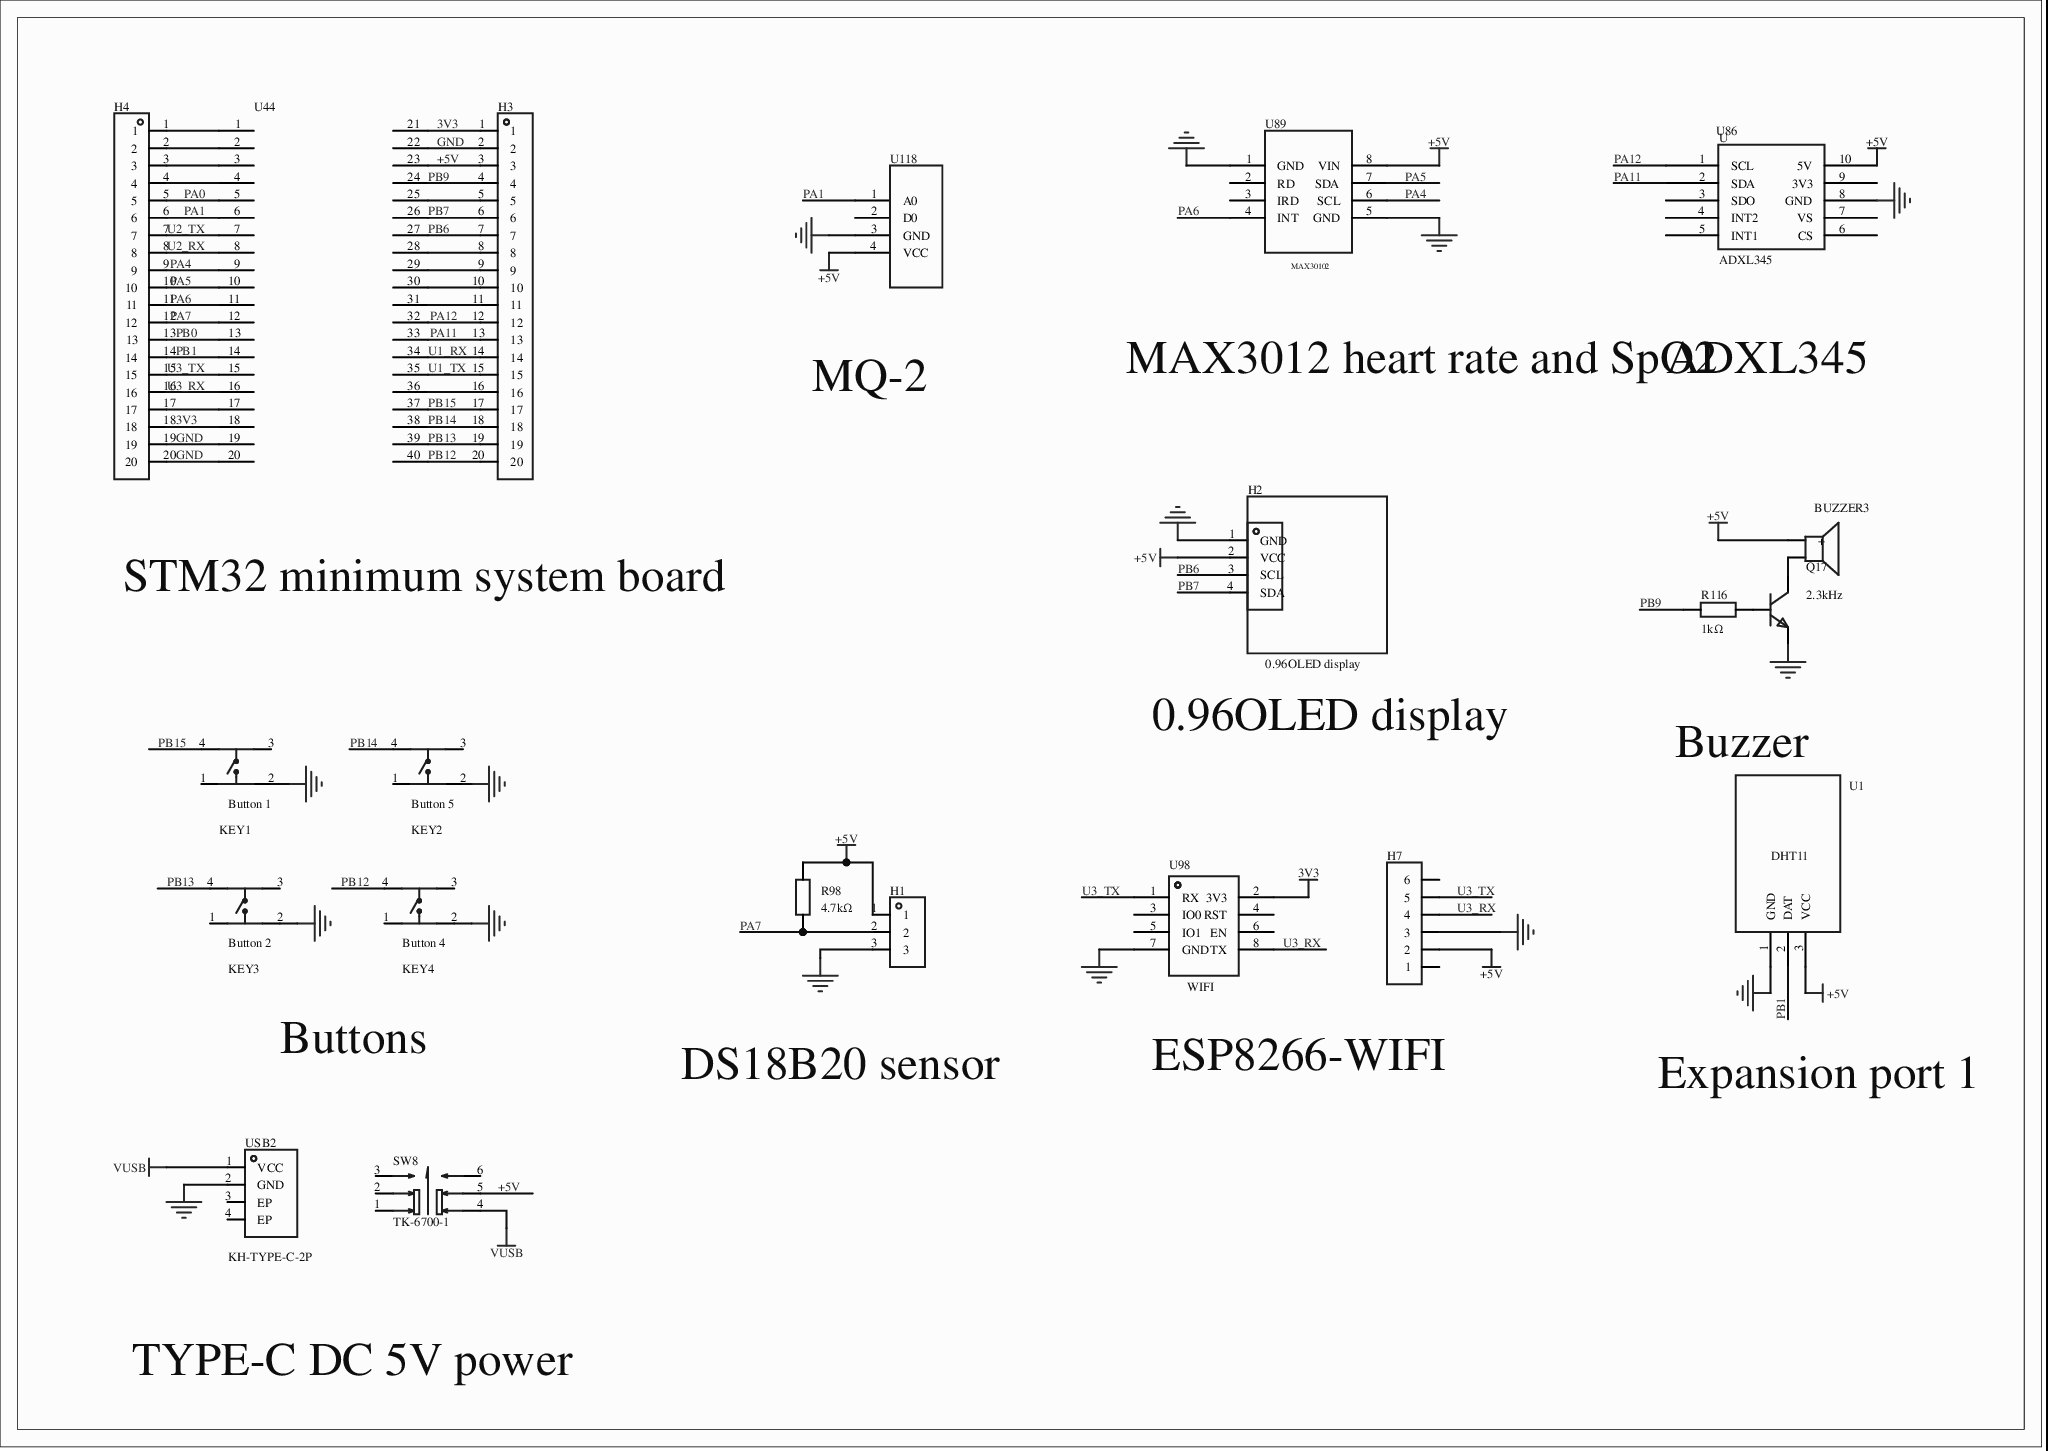
[diagram p0: MISC51907-2.schdoc]
# Altium project MISC51907-3.PrjPcb
1 sheet, 21 parts. Net scope: global (net labels, ports and power ports of the same name join across sheets).
Board file: MISC51907.pcbdoc

## Sheet MISC51907-2.schdoc
size 297 x 210 mm; @Project Name: MISC51907; @Page Count: 1; @Update Date: 2026-04-23; @Create Date: 2026-04-23; @Schematic Name: MISC51907; @Page No: 1; @Board Name: MISC51907; @Create Time: 11:51:39; @Update Time: 11:51:40

### Parts
BUZZER3  2.3kHz  [BUZ-TH_BD12.0-P7.60-D0.6-FD]
H1  (no value)  [HDR-TH_3P-P2.54-V-F]
H2  2.54-1*4P female  [HDR-TH_4P-P2.54-V-F]  (value not drawn)
H3  (no value)  [HDR-TH_20P-P2.54-V-M-1]
H4  (no value)  [HDR-TH_20P-P2.54-V-M-1]
H7  (no value)  [HDR-TH_6P-P2.54-V-M-1]
KEY1  Button 1  [KEY-TH_4P-L6.0-W6.0-P4.50-LS7.5]
KEY2  Button 5  [KEY-TH_4P-L6.0-W6.0-P4.50-LS7.5]
KEY3  Button 2  [KEY-TH_4P-L6.0-W6.0-P4.50-LS7.5]
KEY4  Button 4  [KEY-TH_4P-L6.0-W6.0-P4.50-LS7.5]
Q17  (no value)  [S8050_TO_92]
R98  4.7kΩ  [Res_1/4W]
R116  1kΩ  [Res_1/4W]
SW8  TK-6700-1  [SW-TH_TK-6700-1]
U1  (no value)  [温湿度]
U44  (no value)  [STM32最小系统板]
U86  (no value)  [ADXL345]
U89  (no value)  [MAX30102]
U98  (no value)  [WiFi封装]
U118  (no value)  [MQ-X插件]
USB2  KH-TYPE-C-2P  [USB-SMD_KH-TYPE-C-2P]

### Nets
3V3: H3.1 H4.18 U44.18 U44.21 U98.2(3V3)
+5V: BUZZER3.1(+) H1.1 H2.2(VCC) H3.3 H7.2 R98.2 SW8.5 U1.3(VCC) U44.23 U86.10(5V) U89.8(VIN) U118.4(VCC)
GND: H1.3 H2.1(GND) H3.2 H4.19 H4.20 H7.3 KEY1.2 KEY2.2 KEY3.2 KEY4.2 Q17.1(E) U1.1(GND) U44.19 U44.20 U44.22 U86.8(GND) U89.1(GND) U89.5(GND) U98.7(GND) U118.3(GND) USB2.2(GND)
VUSB: SW8.4 USB2.1(VCC)
PA0: H4.5 U44.5
PA1: H4.6 U44.6 U118.1(A0)
PA4: H4.9 U44.9 U89.6(SCL)
PA5: H4.10 U44.10 U89.7(SDA)
PA6: H4.11 U44.11 U89.4(INT)
PA7: H1.2 H4.12 R98.1 U44.12
PA11: H3.13 U44.33 U86.2(SDA)
PA12: H3.12 U44.32 U86.1(SCL)
PB0: H4.13 U44.13
PB1: H4.14 U1.2(DAT) U44.14
PB6: H2.3(SCL) H3.7 U44.27
PB7: H2.4(SDA) H3.6 U44.26
PB9: H3.4 R116.1 U44.24
PB12: H3.20 KEY4.4 U44.40
PB13: H3.19 KEY3.4 U44.39
PB14: H3.18 KEY2.4 U44.38
PB15: H3.17 KEY1.4 U44.37
U1_RX: H3.14 U44.34
U1_TX: H3.15 U44.35
U2_RX: H4.8 U44.8
U2_TX: H4.7 U44.7
U3_RX: H4.16 H7.4 U44.16 U98.8(TX)
U3_TX: H4.15 H7.5 U44.15 U98.1(RX)
NetBUZZER3_2: BUZZER3.2 Q17.3(C)
NetH3_5: H3.5 U44.25
NetH3_8: H3.8 U44.28
NetH3_9: H3.9 U44.29
NetH3_10: H3.10 U44.30
NetH3_11: H3.11 U44.31
NetH3_16: H3.16 U44.36
NetH4_1: H4.1 U44.1
NetH4_2: H4.2 U44.2
NetH4_3: H4.3 U44.3
NetH4_4: H4.4 U44.4
NetH4_17: H4.17 U44.17
NetQ17_2: Q17.2(B) R116.2

Not connected (* = marked no-connect by the designer): H7 1 6; KEY1 1 3*; KEY2 1 3*; KEY3 1 3*; KEY4 1 3*; SW8 1* 2* 3* 6*; U86 3(SDO) 4(INT2) 5(INT1) 6(CS) 7(VS) 9(3V3); U89 2(RD) 3(IRD); U98 3(IO0) 4(RST) 5(IO1) 6(EN); U118 2(D0); USB2 3(EP) 4(EP)

### Notes on the sheet
- MQ-2
- MAX3012 heart rate and SpO2
- ADXL345
- STM32 minimum system board
- 0.96OLED display
- Buzzer
- Buttons
- DS18B20 sensor
- ESP8266-WIFI
- Expansion port 1
- TYPE-C DC 5V power

### Library data of the parts
BUZZER3 = TMB12A05_C96093: 驱动方式:有源(内含驱动线路);构造类型:电磁式;额定电压:5V;频率:2.3kHz;声压(SPL):85dB@5V,10cm;; Manufacturer: 华能; AddInBom: yes; ModelId: 16ab50e14c5b4f2c986c135bdba60e37; ModelName: BUZ-TH_D12.0-H9.5-P7.60; ModelTransform: 472.44,472.176,0,90,0,0,-0.787,0,-177.165; Oscillator Circuit: Active (with built-in driver circuit); Technology Type: Electromagnetic; Rated Voltage: 5V; Operating Voltage: 4V~8V; Device: TMB12A05_C96093; Symbol: TMB12A05; LCSC Part Name: TMB12A05; SupplierPart: C96093; ManufacturerPart: TMB12A05; Supplier Footprint: 插件,D=12mm; JLCPCB Part Class: Extended Part; Datasheet: https://example.com/20170522/1495448324811.pdf; Supplier: LCSC; ConvertToPcb: yes; FootprintName: BUZ-TH_BD12.0-P7.60-D0.6-FD; Value: 2.3kHz; Sound Pressure Level (SPL): 85dB@5V,10cm; Diameter (φD): 12mm; Height: 9.8mm
H1 = HDR-F_2.54_1x3P: Symbol: PM254V-11-03-H85; ConvertToPcb: yes; ModelId: f3b3cc5aae9641bf9e56fc160cef875b0819f05c4eef4c71ace90d822a990e87; ModelName: HDR2.54-F-LI-1X3P; ModelTransform: 299.9994,100,0,0,0,0,0,0,-118.11; Device: HDR-F_2.54_1x3P; AddInBom: yes; SupplierPart: C541850; Supplier Footprint: 插件; FootprintName: HDR-TH_3P-P2.54-V-F
H2 = 0.96OLED屏幕: 插孔结构:1x4P;间距:2.54mm;行距:-;圆孔/方孔:方孔;安装类型:直插;排数:单排;总孔位数:4P;额定电流:3A;额定电压:-;插孔方向:顶部;塑高:-;触头材质:青铜;触头镀层:-;工作温度范围:-40℃~+105℃;焊接温度(最大值):-;; Manufacturer: BOOMELE(博穆精密); ManufacturerPart: 2.54-1*4P母; Device: 0.96OLED display; AddInBom: yes; Holes Structure: 1x4P; Pitch: 2.54mm; Circular Hole / Square Hole: Square; Number of Holes: 4P; Current Rating (Max): 3A; Holes Direction: Top; ModelId: 57daaad411c24bd7bd5d06edf5c4d16b; ModelName: HDR-TH_4P-P2.54-F-LI-1X4P; ModelTransform: 415.7472,98.425,0,0,0,0,0,0,-118.11; Supplier: LCSC; SupplierPart: C2718488; JLCPCB Part Class: Extended library; LCSC Part Name: 间距:2.54mm 1x4P 直插; Supplier Footprint: 插件,P=2.54mm; Datasheet: https://example.com/20210301/C2718488_F4427B881E42CAA8DDB0B1C12B3A522C.pdf; ConvertToPcb: yes; Row Spacing: -; Mounting Type: Through-hole; Number of Rows: Single row; Voltage Rating (Max): -; Insulation Height: -; Contact Material: Bronze; Contact Plating: -; Operating Temperature Range: -40℃~+105℃; Soldering Temperature(Max): -; SymbolName: 0.96OLED display; FootprintName: HDR-TH_4P-P2.54-V-F
H3 H4 = HDR-M_2.54_1x20P: 间距:2.54mm;总PIN位数:20;排数:1;插针结构:-;行距:-;安装类型:直插;圆针/方针:-;额定电流:-;额定电压:-;配合针长度:-;塑高:-;触头材质:黄铜;触头镀层:-;颜色:黑色;; Symbol: HDR_2.54-1x20P; ConvertToPcb: yes; ModelId: f68709be121d406db68b06f32a595389; ModelName: HDR-M-2.54_1x20; ModelTransform: 1999.996,100,0,0,0,0,0,0,-118.11; Device: HDR-M_2.54_1x20P; AddInBom: yes; SupplierPart: C50981; Supplier Footprint: 插件; FootprintName: HDR-TH_20P-P2.54-V-M-1
H7 = HDR-M_2.54_1x6P: Symbol: Header-Male-2.54_1x6; ConvertToPcb: yes; ModelId: 60739dffc9b04830a286435b0fefbd4a; ModelName: HDR2.54-M-LI-1X6P; ModelTransform: 599.999,100,0,0,0,0,0,0,-118.11; Device: HDR-M_2.54_1x6P; AddInBom: yes; SupplierPart: C37208; Supplier Footprint: 插件; FootprintName: HDR-TH_6P-P2.54-V-M-1
KEY1 = 按键开关6*6*8: 电路结构:SPST;触点额定电流:-;按钮头类型:Round Button;按钮作用方向:Top Actuated;; Manufacturer Part: 按键1; Device: Tact switch 6*6*8; Symbol: button6*6*8; AddInBom: yes; ModelId: 84d39232fe0a426fa95ea2653754a6e5; ModelName: KEY-TH_4P-L6.0-W6.0-H4.5-LS6.5-P4.5; ModelTransform: 306.868,236.22,0,0,0,0,0,0,-118.11; LCSC Part Name: 按键开关6*6*8   直插; SupplierPart: C59982; Supplier Footprint: Through Hole; JLCPCB Part Class: Extended library; Datasheet: https://example.com/20151126/1457707591845.pdf; Supplier: LCSC; ConvertToPcb: yes; FootprintName: KEY-TH_4P-L6.0-W6.0-P4.50-LS7.5
KEY2 = 按键开关6*6*8: 电路结构:SPST;触点额定电流:-;按钮头类型:Round Button;按钮作用方向:Top Actuated;; Manufacturer Part: 按键5; Device: Tact switch 6*6*8; Symbol: button6*6*8; AddInBom: yes; ModelId: 84d39232fe0a426fa95ea2653754a6e5; ModelName: KEY-TH_4P-L6.0-W6.0-H4.5-LS6.5-P4.5; ModelTransform: 306.868,236.22,0,0,0,0,0,0,-118.11; LCSC Part Name: 按键开关6*6*8   直插; SupplierPart: C59982; Supplier Footprint: Through Hole; JLCPCB Part Class: Extended library; Datasheet: https://example.com/20151126/1457707591845.pdf; Supplier: LCSC; ConvertToPcb: yes; FootprintName: KEY-TH_4P-L6.0-W6.0-P4.50-LS7.5
KEY3 = 按键开关6*6*8: 电路结构:SPST;触点额定电流:-;按钮头类型:Round Button;按钮作用方向:Top Actuated;; Manufacturer Part: 按键2; Device: Tact switch 6*6*8; Symbol: button6*6*8; AddInBom: yes; ModelId: 84d39232fe0a426fa95ea2653754a6e5; ModelName: KEY-TH_4P-L6.0-W6.0-H4.5-LS6.5-P4.5; ModelTransform: 306.868,236.22,0,0,0,0,0,0,-118.11; LCSC Part Name: 按键开关6*6*8   直插; SupplierPart: C59982; Supplier Footprint: Through Hole; JLCPCB Part Class: Extended library; Datasheet: https://example.com/20151126/1457707591845.pdf; Supplier: LCSC; ConvertToPcb: yes; FootprintName: KEY-TH_4P-L6.0-W6.0-P4.50-LS7.5
KEY4 = 按键开关6*6*8: 电路结构:SPST;触点额定电流:-;按钮头类型:Round Button;按钮作用方向:Top Actuated;; Manufacturer Part: 按键4; Device: Tact switch 6*6*8; Symbol: button6*6*8; AddInBom: yes; ModelId: 84d39232fe0a426fa95ea2653754a6e5; ModelName: KEY-TH_4P-L6.0-W6.0-H4.5-LS6.5-P4.5; ModelTransform: 306.868,236.22,0,0,0,0,0,0,-118.11; LCSC Part Name: 按键开关6*6*8   直插; SupplierPart: C59982; Supplier Footprint: Through Hole; JLCPCB Part Class: Extended library; Datasheet: https://example.com/20151126/1457707591845.pdf; Supplier: LCSC; ConvertToPcb: yes; FootprintName: KEY-TH_4P-L6.0-W6.0-P4.50-LS7.5
Q17 = S8050_TO_NPN: ConvertToPcb: yes; ModelId: aafe8e06f2154e7c93506efd0d6632dd; ModelName: TO-92-3_L4.9-W3.7-P1.27-L; ModelTransform: 180.78,141.44,417.3,0,0,0,0,0,-200; Device: S8050_TO_NPN; AddInBom: yes; Supplier Footprint: TO-92; SymbolName: S8050_TO_NPN; FootprintName: S8050_TO_92
R98 R116 = Res_AXIAL-1/4W: Symbol: Resistor; AddInBom: yes; ModelId: 463263665006444ab7a47bd11b0cf956; ModelName: RES-TH_BD2.4-L6.3-P10.30-D0.6; ModelTransform: 427.165,94.32816,0,0,0,0,0,0,-196.85; Device: Res_AXIAL-1/4W; Supplier Footprint: 轴向引线; ConvertToPcb: yes; FootprintName: Res_1/4W
  R98: Value: 4.7kΩ
  R116: Value: 1kΩ
SW8 = TK-6700-1: Manufacturer: Yuandi(元迪); AddInBom: yes; ModelId: 1dccfbf2ceb24a728093c1f6ee61932a; ModelTransform: 275.59,275.59,0,90,0,0,0,0,-137.795; Device: TK-6700-1; Symbol: TK-6700-1; LCSC Part Name: 自锁开关7*7*12.7有声有锁高导高柄插件双排6P按键开关带锁DIP六脚; SupplierPart: C528782; ManufacturerPart: TK-6700-1; Supplier Footprint: 插件; JLCPCB Part Class: Extended Part; Datasheet: https://example.com/20200831/C528782_58F076EBF84BD8A9E2DE38DB1C0986D4.pdf; Supplier: LCSC; ConvertToPcb: yes; FootprintName: SW-TH_TK-6700-1; ModelName: SW-TH_TK-6700-1
U1 = 温湿度DHT11: Device: Temperature and humidity DHT11; AddInBom: yes; Symbol: Temperature and humidity DHT11; ConvertToPcb: yes; FootprintName: Temp-humidity
U44 = STM32最小系统板: Device: STM32 minimum system board; AddInBom: yes; ConvertToPcb: yes; SymbolName: STM32 minimum system board; FootprintName: STM32 minimum system board
U86 = ADXL345: AddInBom: yes; Device: ADXL345; ConvertToPcb: yes; SymbolName: ADXL345; FootprintName: ADXL345
U89 = MAX30102: AddInBom: yes; Device: MAX30102; ConvertToPcb: yes; SymbolName: MAX30102; FootprintName: MAX30102
U98 = WiFi模块: Device: WiFi module; AddInBom: yes; ConvertToPcb: yes; SymbolName: WiFi module; FootprintName: WiFi footprint
U118 = MQ-X插件: Device: MQ-X plug-in; AddInBom: yes; Symbol: MQ-X plug-in; ConvertToPcb: yes; FootprintName: MQ-X plug-in
USB2 = KH-TYPE-C-2P: 连接器类型:Type-C;标准:-;公母:-;端口数量:-;触点数量:2P;安装方式:-;额定电流 - 电源:-;触头材质:-;触头镀层:-;工作温度范围:-;; Manufacturer: kinghelm(金航标); AddInBom: yes; ModelId: 4464b34a7d0f48c2b8c2350e914c93f5; ModelTransform: 352.362,255.31449,0,0,0,0,0,-49.213,-98.425; Connector Type: Type-C; Number of Contacts: 2P; Symbol: KH-TYPE-C-2P; Device: KH-TYPE-C-2P; LCSC Part Name: Type-C; SupplierPart: C2919656; ManufacturerPart: KH-TYPE-C-2P; Supplier Footprint: 插件; JLCPCB Part Class: Extended Part; Datasheet: https://example.com/20220707/620587A9E0589B27D96D3CEE595CBC98.pdf; Supplier: LCSC; ConvertToPcb: yes; FootprintName: USB-SMD_KH-TYPE-C-2P; ModelName: USB-SMD_KH-TYPE-C-2P; Standard: -; Gender: -; Number of Ports: -; Mounting Style: -; Current Rating - Power (Max): -; Contact Material: -; Contact Plating: -; Operating Temperature Range: -